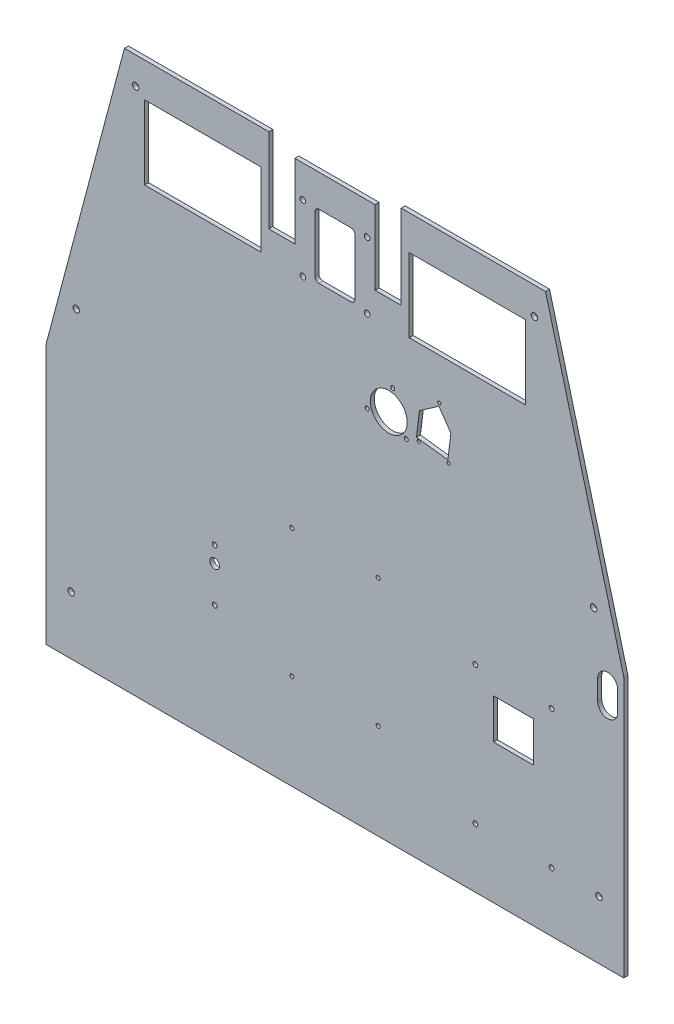
from build123d import *

# Parameters (mm, degrees)
BOSS_EXTRUDE1_DEPTH  = 10
SKETCH2_R            = 8
CUT_EXTRUDE1_DEPTH   = 10
LPATTERN1_COUNT      = 2
LPATTERN1_PITCH      = 1316
SKETCH3_R            = 8
CUT_EXTRUDE2_DEPTH   = 10
LPATTERN2_COUNT      = 2
LPATTERN2_PITCH      = 1290
SKETCH4_R            = 8
CUT_EXTRUDE3_DEPTH   = 10
LPATTERN3_COUNT      = 2
LPATTERN3_PITCH      = 994
CUT_EXTRUDE4_DEPTH   = 10
SKETCH6_W            = 100
SKETCH6_H            = 100
CUT_EXTRUDE5_DEPTH   = 10
SKETCH7_R            = 6
CUT_EXTRUDE6_DEPTH   = 10
LPATTERN4_COUNT      = 2
LPATTERN4_PITCH      = 190
LPATTERN4_COUNT_DIR2 = 2
LPATTERN4_PITCH_DIR2 = 344
SKETCH8_R            = 5
CUT_EXTRUDE7_DEPTH   = 10
LPATTERN5_COUNT      = 2
LPATTERN5_PITCH      = 320
LPATTERN5_COUNT_DIR2 = 2
LPATTERN5_PITCH_DIR2 = 215
SKETCH9_W            = 290
SKETCH9_H            = 184
CUT_EXTRUDE8_DEPTH   = 10
SKETCH10_W           = 100
SKETCH10_H           = 160
CUT_EXTRUDE9_DEPTH   = 10
FILLET1_R            = 10
SKETCH11_R           = 7
CUT_EXTRUDE10_DEPTH  = 10
LPATTERN7_COUNT      = 2
LPATTERN7_PITCH      = 160
LPATTERN7_COUNT_DIR2 = 2
LPATTERN7_PITCH_DIR2 = 165
SKETCH12_R           = 5
CUT_EXTRUDE11_DEPTH  = 10
SKETCH14_R           = 46
CUT_EXTRUDE12_DEPTH  = 10
SKETCH15_R           = 5
CUT_EXTRUDE13_DEPTH  = 10
LPATTERN8_COUNT      = 2
LPATTERN8_PITCH      = 99
SKETCH16_R           = 4
CUT_EXTRUDE14_DEPTH  = 10
CUT_EXTRUDE15_DEPTH  = 10
SKETCH18_R           = 4
CUT_EXTRUDE16_DEPTH  = 10
LPATTERN9_COUNT      = 2
LPATTERN9_PITCH      = 75
SKETCH19_R           = 6
CUT_EXTRUDE17_DEPTH  = 10
LPATTERN10_COUNT     = 2
LPATTERN10_PITCH     = 130
SKETCH20_R           = 12
CUT_EXTRUDE18_DEPTH  = 10
LPATTERN11_COUNT     = 2
LPATTERN11_PITCH     = 660
SKETCH21_W           = 65
SKETCH21_H           = 210
CUT_EXTRUDE19_DEPTH  = 10
SKETCH22_W           = 65
SKETCH22_H           = 210
CUT_EXTRUDE20_DEPTH  = 10
SKETCH23_W           = 200
SKETCH23_H           = 25
CUT_EXTRUDE21_DEPTH  = 10


with BuildPart() as part:
    # Sketch1 → Boss-Extrude1 (new body)
    with BuildSketch(Plane.XY):
        Polygon((-720, 0), (720, 0), (720, 650), (525, 1385), (-525, 1385), (-720, 650), align=None)
    extrude(amount=BOSS_EXTRUDE1_DEPTH)

    # Sketch2 → Cut-Extrude1 (cut)
    with BuildSketch(Plane.XY.offset(10)):
        with Locations((-658, 145)):
            Circle(SKETCH2_R)
    cut_extrude1 = extrude(amount=-CUT_EXTRUDE1_DEPTH, mode=Mode.SUBTRACT)

    # LPattern1: Cut-Extrude1 ×2
    with Locations(*[(i * LPATTERN1_PITCH, 0, 0) for i in range(1, LPATTERN1_COUNT)]):
        add(cut_extrude1, mode=Mode.SUBTRACT)

    # Sketch3 → Cut-Extrude2 (cut)
    with BuildSketch(Plane.XY.offset(10)):
        with Locations((-645, 762)):
            Circle(SKETCH3_R)
    cut_extrude2 = extrude(amount=-CUT_EXTRUDE2_DEPTH, mode=Mode.SUBTRACT)

    # LPattern2: Cut-Extrude2 ×2
    with Locations(*[(i * LPATTERN2_PITCH, 0, 0) for i in range(1, LPATTERN2_COUNT)]):
        add(cut_extrude2, mode=Mode.SUBTRACT)

    # Sketch4 → Cut-Extrude3 (cut)
    with BuildSketch(Plane.XY.offset(10)):
        with Locations((-497, 1317)):
            Circle(SKETCH4_R)
    cut_extrude3 = extrude(amount=-CUT_EXTRUDE3_DEPTH, mode=Mode.SUBTRACT)

    # LPattern3: Cut-Extrude3 ×2
    with Locations(*[(i * LPATTERN3_PITCH, 0, 0) for i in range(1, LPATTERN3_COUNT)]):
        add(cut_extrude3, mode=Mode.SUBTRACT)

    # Sketch5 → Cut-Extrude4 (cut)
    with BuildSketch(Plane.XY.offset(10)):
        with BuildLine():
            Line((655, 615), (655, 565))
            ThreePointArc((655, 565), (680, 540), (705, 565))
            Line((705, 565), (705, 615))
            ThreePointArc((705, 615), (680, 640), (655, 615))
        make_face()
    extrude(amount=-CUT_EXTRUDE4_DEPTH, mode=Mode.SUBTRACT)

    # Sketch6 → Cut-Extrude5 (cut)
    with BuildSketch(Plane.XY.offset(10)):
        with Locations((445, 397)):
            Rectangle(SKETCH6_W, SKETCH6_H)
    extrude(amount=-CUT_EXTRUDE5_DEPTH, mode=Mode.SUBTRACT)

    # Sketch7 → Cut-Extrude6 (cut)
    with BuildSketch(Plane.XY.offset(10)):
        with Locations((540, 492)):
            Circle(SKETCH7_R)
    cut_extrude6 = extrude(amount=-CUT_EXTRUDE6_DEPTH, mode=Mode.SUBTRACT)

    # LPattern4: Cut-Extrude6 2 × 2
    with Locations(*[(-i * LPATTERN4_PITCH, -j * LPATTERN4_PITCH_DIR2, 0) for i in range(LPATTERN4_COUNT) for j in range(LPATTERN4_COUNT_DIR2) if (i, j) != (0, 0)]):
        add(cut_extrude6, mode=Mode.SUBTRACT)

    # Sketch8 → Cut-Extrude7 (cut)
    with BuildSketch(Plane.XY.offset(10)):
        with Locations((107.5, 238)):
            Circle(SKETCH8_R)
    cut_extrude7 = extrude(amount=-CUT_EXTRUDE7_DEPTH, mode=Mode.SUBTRACT)

    # LPattern5: Cut-Extrude7 2 × 2
    with Locations(*[(-j * LPATTERN5_PITCH_DIR2, i * LPATTERN5_PITCH, 0) for i in range(LPATTERN5_COUNT) for j in range(LPATTERN5_COUNT_DIR2) if (i, j) != (0, 0)]):
        add(cut_extrude7, mode=Mode.SUBTRACT)

    # Sketch9 → Cut-Extrude8 (cut)
    with BuildSketch(Plane.XY.offset(10)):
        with Locations((-330, 1207)):
            Rectangle(SKETCH9_W, SKETCH9_H)
    cut_extrude8 = extrude(amount=-CUT_EXTRUDE8_DEPTH, mode=Mode.SUBTRACT)

    # Sketch10 → Cut-Extrude9 (cut)
    with BuildSketch(Plane.XY.offset(10)):
        with Locations((0, 1200)):
            Rectangle(SKETCH10_W, SKETCH10_H)
    extrude(amount=-CUT_EXTRUDE9_DEPTH, mode=Mode.SUBTRACT)

    # Fillet1
    fillet1_edges = [part.edges().sort_by_distance(p)[0] for p in [
        (-50, 1120, 5),
        (-50, 1280, 5),
        (50, 1280, 5),
        (50, 1120, 5),
    ]]
    fillet(fillet1_edges, radius=FILLET1_R)

    # Sketch11 → Cut-Extrude10 (cut)
    with BuildSketch(Plane.XY.offset(10)):
        with Locations((80, 1280)):
            Circle(SKETCH11_R)
    cut_extrude10 = extrude(amount=-CUT_EXTRUDE10_DEPTH, mode=Mode.SUBTRACT)

    # LPattern7: Cut-Extrude10 2 × 2
    with Locations(*[(-i * LPATTERN7_PITCH, -j * LPATTERN7_PITCH_DIR2, 0) for i in range(LPATTERN7_COUNT) for j in range(LPATTERN7_COUNT_DIR2) if (i, j) != (0, 0)]):
        add(cut_extrude10, mode=Mode.SUBTRACT)

    # Sketch12 → Cut-Extrude11 (cut)
    with BuildSketch(Plane.XY.offset(10)):
        with Locations((144, 986)):
            Circle(SKETCH12_R)
    extrude(amount=-CUT_EXTRUDE11_DEPTH, mode=Mode.SUBTRACT)

    # Sketch14 → Cut-Extrude12 (cut)
    with BuildSketch(Plane.XY.offset(10)):
        with Locations((134.067324237, 929.668996528)):
            Circle(SKETCH14_R)
    extrude(amount=-CUT_EXTRUDE12_DEPTH, mode=Mode.SUBTRACT)

    # Sketch15 → Cut-Extrude13 (cut)
    with BuildSketch(Plane.XY.offset(10)):
        with Locations((80.318272947, 909.902118035)):
            Circle(SKETCH15_R)
    cut_extrude13 = extrude(amount=-CUT_EXTRUDE13_DEPTH, mode=Mode.SUBTRACT)

    # LPattern8: Cut-Extrude13 ×2
    with Locations(*[Vector(0.9848077530122089, -0.17364817766692592, 0) * (i * LPATTERN8_PITCH) for i in range(1, LPATTERN8_COUNT)]):
        add(cut_extrude13, mode=Mode.SUBTRACT)

    # Sketch16 → Cut-Extrude14 (cut)
    with BuildSketch(Plane.XY.offset(10)):
        with Locations((260, 1012)):
            Circle(SKETCH16_R)
    extrude(amount=-CUT_EXTRUDE14_DEPTH, mode=Mode.SUBTRACT)

    # Sketch17 → Cut-Extrude15 (cut)
    with BuildSketch(Plane.XY.offset(10)):
        Polygon((259.025045253, 1004.059630787), (210.570516199, 970.471558288), (203.044210897, 909.174720581), (281.455356876, 899.547042452), (288.981662179, 960.843880159), align=None)
    extrude(amount=-CUT_EXTRUDE15_DEPTH, mode=Mode.SUBTRACT)

    # Sketch18 → Cut-Extrude16 (cut)
    with BuildSketch(Plane.XY.offset(10)):
        with Locations((208.764544822, 902.427292939)):
            Circle(SKETCH18_R)
    cut_extrude16 = extrude(amount=-CUT_EXTRUDE16_DEPTH, mode=Mode.SUBTRACT)

    # LPattern9: Cut-Extrude16 ×2
    with Locations(*[Vector(0.9925461516413229, -0.12186934340514104, 0) * (i * LPATTERN9_PITCH) for i in range(1, LPATTERN9_COUNT)]):
        add(cut_extrude16, mode=Mode.SUBTRACT)

    # Sketch19 → Cut-Extrude17 (cut)
    with BuildSketch(Plane.XY.offset(10)):
        with Locations((-300, 295)):
            Circle(SKETCH19_R)
    cut_extrude17 = extrude(amount=-CUT_EXTRUDE17_DEPTH, mode=Mode.SUBTRACT)

    # LPattern10: Cut-Extrude17 ×2
    with Locations(*[(0, i * LPATTERN10_PITCH, 0) for i in range(1, LPATTERN10_COUNT)]):
        add(cut_extrude17, mode=Mode.SUBTRACT)

    # Sketch20 → Cut-Extrude18 (cut)
    with BuildSketch(Plane.XY.offset(10)):
        with Locations((-300, 385)):
            Circle(SKETCH20_R)
    extrude(amount=-CUT_EXTRUDE18_DEPTH, mode=Mode.SUBTRACT)

    # LPattern11: Cut-Extrude8 ×2
    with Locations(*[(i * LPATTERN11_PITCH, 0, 0) for i in range(1, LPATTERN11_COUNT)]):
        add(cut_extrude8, mode=Mode.SUBTRACT)

    # Sketch21 → Cut-Extrude19 (cut)
    with BuildSketch(Plane.XY.offset(10)):
        with Locations((132.5, 1280)):
            Rectangle(SKETCH21_W, SKETCH21_H)
    extrude(amount=-CUT_EXTRUDE19_DEPTH, mode=Mode.SUBTRACT)

    # Sketch22 → Cut-Extrude20 (cut)
    with BuildSketch(Plane.XY.offset(10)):
        with Locations((-132.5, 1280)):
            Rectangle(SKETCH22_W, SKETCH22_H)
    extrude(amount=-CUT_EXTRUDE20_DEPTH, mode=Mode.SUBTRACT)

    # Sketch23 → Cut-Extrude21 (cut)
    with BuildSketch(Plane.XY.offset(10)):
        with Locations((0, 1372.5)):
            Rectangle(SKETCH23_W, SKETCH23_H)
    extrude(amount=-CUT_EXTRUDE21_DEPTH, mode=Mode.SUBTRACT)


solid = part.part
